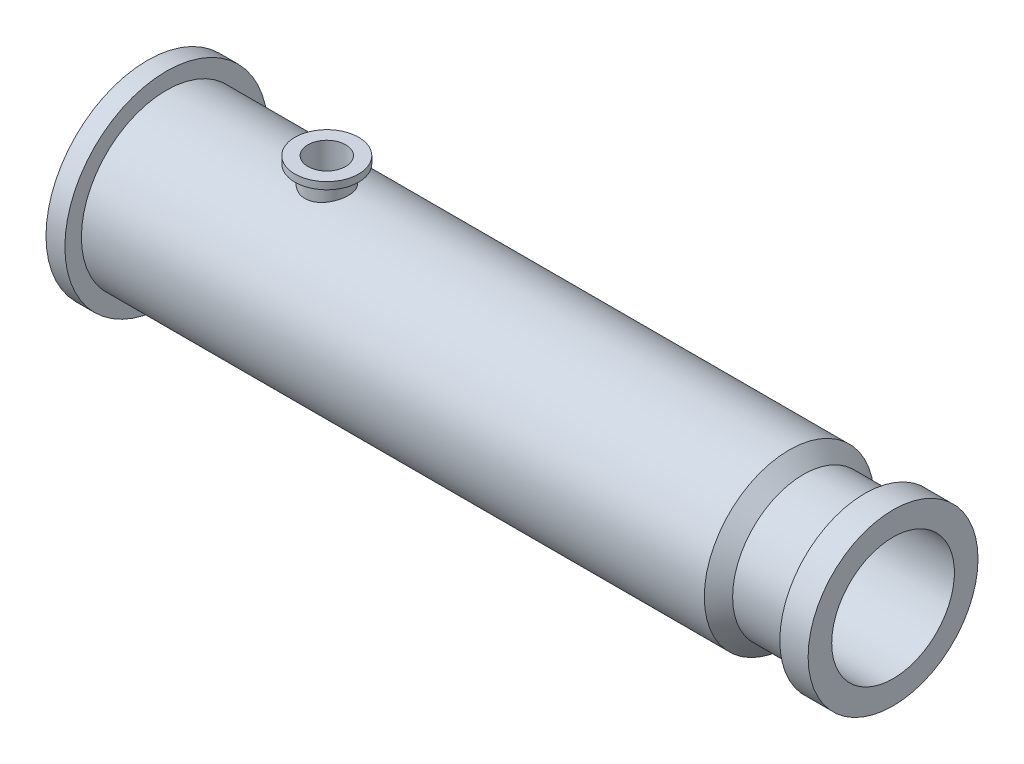
from build123d import *

# Parameters (mm, degrees)
SKETCH3_R           = 46
SKETCH3_R_2         = 40
BOSS_EXTRUDE1_DEPTH = 215
SKETCH4_R           = 160
CUT_EXTRUDE1_DEPTH  = 900
CUT_EXTRUDE2_START  = -300
SKETCH5_R           = 40
CUT_EXTRUDE2_DEPTH  = 300
SKETCH6_R           = 67.5
SKETCH6_R_2         = 40
BOSS_EXTRUDE2_DEPTH = 15


with BuildPart() as part:
    # Sketch1 → Revolve1 (revolve)
    with BuildSketch(Plane.XY, mode=Mode.PRIVATE) as revolve1_sk:
        Polygon((0, 160), (0, 215), (40, 215), (40, 180), (1360, 180), (1390, 150), (1520, 150), (1520, 180), (1580, 180), (1580, 130), (1381.715728753, 130), (1351.715728753, 160), align=None)
    revolve(revolve1_sk.sketch.rotate(Axis((0, 0, 0), (1, 0, 0)), 90), axis=Axis((0, 0, 0), (1, 0, 0)))

    # Sketch3 → Boss-Extrude1 (add)
    with BuildSketch(Plane(origin=(0, 0, 0), x_dir=(1, 0, 0), z_dir=(0, 1, 0))):
        with Locations(Location((380, 0, 0), (0, 0, 90))):
            Circle(SKETCH3_R)
        with Locations(Location((380, 0, 0), (0, 0, 90))):
            Circle(SKETCH3_R_2, mode=Mode.SUBTRACT)
    extrude(amount=BOSS_EXTRUDE1_DEPTH)

    # Sketch4 → Cut-Extrude1 (cut)
    with BuildSketch(Plane.ZY):
        Circle(SKETCH4_R)
    extrude(amount=-CUT_EXTRUDE1_DEPTH, mode=Mode.SUBTRACT)

    # Sketch5 → Cut-Extrude2 (cut)
    with BuildSketch(Plane(origin=(0, 215, 0), x_dir=(1, 0, 0), z_dir=(0, 1, 0)).offset(CUT_EXTRUDE2_START)):
        with Locations(Location((380, 0, 0), (0, 0, 270))):
            Circle(SKETCH5_R)
    extrude(amount=CUT_EXTRUDE2_DEPTH, mode=Mode.SUBTRACT)

    # Sketch6 → Boss-Extrude2 (add)
    with BuildSketch(Plane(origin=(0, 215, 0), x_dir=(1, 0, 0), z_dir=(0, 1, 0))):
        with Locations(Location((380, 0, 0), (0, 0, 270))):
            Circle(SKETCH6_R)
        with Locations(Location((380, 0, 0), (0, 0, 270))):
            Circle(SKETCH6_R_2, mode=Mode.SUBTRACT)
    extrude(amount=BOSS_EXTRUDE2_DEPTH)


solid = part.part
